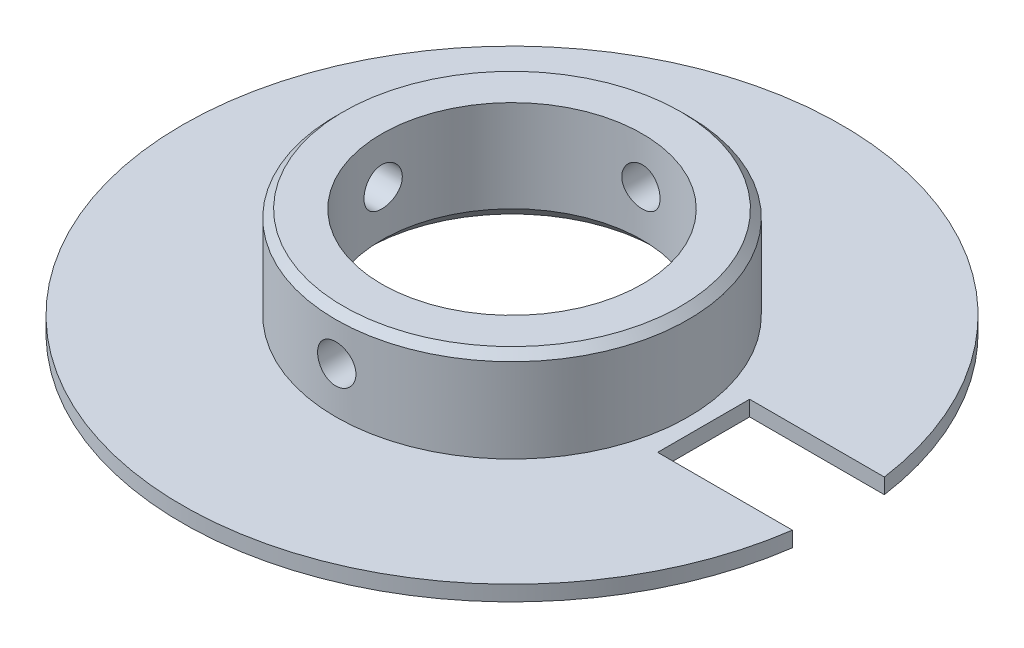
from build123d import *

# Parameters (mm, degrees)
CHAMFER1_SIZE      = 1
SKETCH7_W          = 11.256792451
SKETCH7_H          = 6
CUT_EXTRUDE1_DEPTH = 10
SKETCH9_W          = 1.25
SKETCH9_H          = 21.5
CHAMFER2_SIZE      = 0.5
CIRPATTERN1_COUNT  = 4


with BuildPart() as part:
    # Sketch2 → Revolve1 (revolve)
    with BuildSketch(Plane(origin=(0, 0, 0), x_dir=(0, 0, -1), z_dir=(1, 0, 0)), mode=Mode.PRIVATE) as revolve1_sk:
        Polygon((8.5, 0), (21.5, 0), (21.5, 1), (11.5, 1), (11.5, 7), (8.5, 7), align=None)
    revolve(revolve1_sk.sketch.rotate(Axis((0, 67.294927727, 0), (0, -1, 0)), 180), axis=Axis((0, 67.294927727, 0), (0, -1, 0)))

    # Chamfer1
    chamfer1_edges = [part.edges().sort_by_distance(p)[0] for p in [
        (0, 0, -8.5),
    ]]
    chamfer(chamfer1_edges, length=CHAMFER1_SIZE)

    # Sketch7 → Cut-Extrude1 (cut)
    with BuildSketch(Plane(origin=(0, 1, 0), x_dir=(1, 0, 0), z_dir=(0, 1, 0))):
        with Locations((18.128396226, 0)):
            Rectangle(SKETCH7_W, SKETCH7_H)
    extrude(amount=-CUT_EXTRUDE1_DEPTH, mode=Mode.SUBTRACT)

    # Sketch9 → M3 Tapped Hole2 (revolve, cut)
    with BuildSketch(Plane(origin=(0, 4, 0), x_dir=(0, 0, -1), z_dir=(0, 1, 0))):
        with Locations((0.625, 10.75)):
            Rectangle(SKETCH9_W, SKETCH9_H)
    m3_tapped_hole2 = revolve(axis=Axis((6.35, 4, 0), (-1, 0, 0)), mode=Mode.SUBTRACT)

    # Chamfer2
    chamfer2_edges = [part.edges().sort_by_distance(p)[0] for p in [
        (0, 7, -11.5),
    ]]
    chamfer(chamfer2_edges, length=CHAMFER2_SIZE)

    # CirPattern1: M3 Tapped Hole2 ×4 about axis, 1 skipped
    cirpattern1_axis = Axis((0, 67.294927727, 0), (0, 1, 0))
    add([m3_tapped_hole2.rotate(cirpattern1_axis, i * 360 / CIRPATTERN1_COUNT) for i in range(1, CIRPATTERN1_COUNT) if i not in (2,)], mode=Mode.SUBTRACT)


solid = part.part
